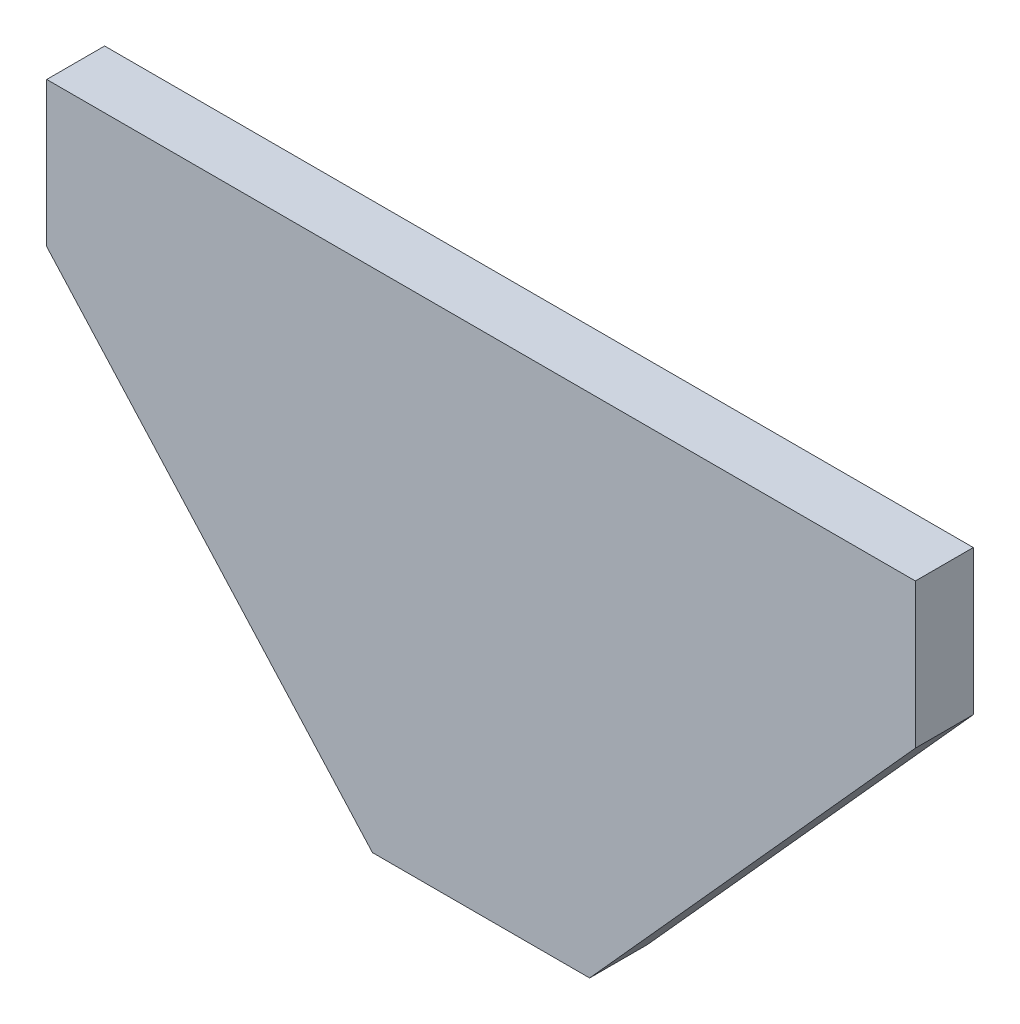
from build123d import *

# Parameters (mm, degrees)
SKETCH1_W           = 120
SKETCH1_H           = 70
BOSS_EXTRUDE1_DEPTH = 8
CUT_EXTRUDE1_DEPTH  = 8


with BuildPart() as part:
    # Sketch1 → Boss-Extrude1 (new body)
    with BuildSketch(Plane.XY):
        Rectangle(SKETCH1_W, SKETCH1_H)
    extrude(amount=BOSS_EXTRUDE1_DEPTH)

    # Sketch2 → Cut-Extrude1 (cut)
    with BuildSketch(Plane.XY.offset(8)):
        Polygon((-60, 15), (-15, -35), (-60, -35), align=None)
        Polygon((15, -35), (60, 15), (60, -35), align=None)
    extrude(amount=-CUT_EXTRUDE1_DEPTH, mode=Mode.SUBTRACT)


solid = part.part
